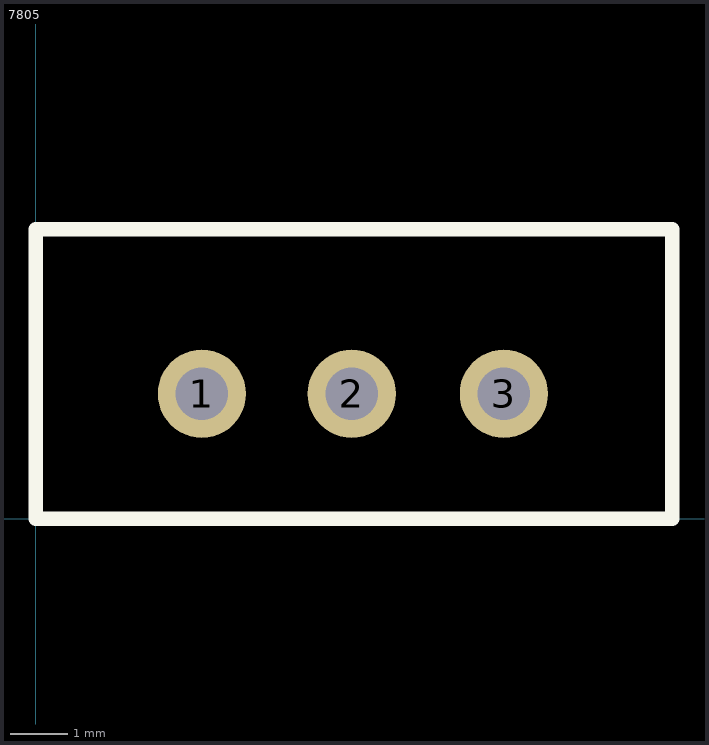
[diagram p0: the footprint, top view; thin cyan lines are the x and y axes]
# Altium footprint library MISC89340-2.PcbLib: 1 footprints
Each footprint in its own frame and in the unit in brackets; x right, y up, seen from the top. Pads: shape width x height; smd on the part's side, far side on the other; paste and mask are expansions set on the pad; w line width, h text height; cw(c..) or ccw(c..) is an arc to the next point about the centre after c.

## 7805 [mil]
pads (3):
  round 60 hole 35.83: 1(113.03,85) 2(215,85) 3(318.5,85)
Top Overlay:
  lines w10: 0,0 433.07,0 433.07,196.85 0,196.85 0,0